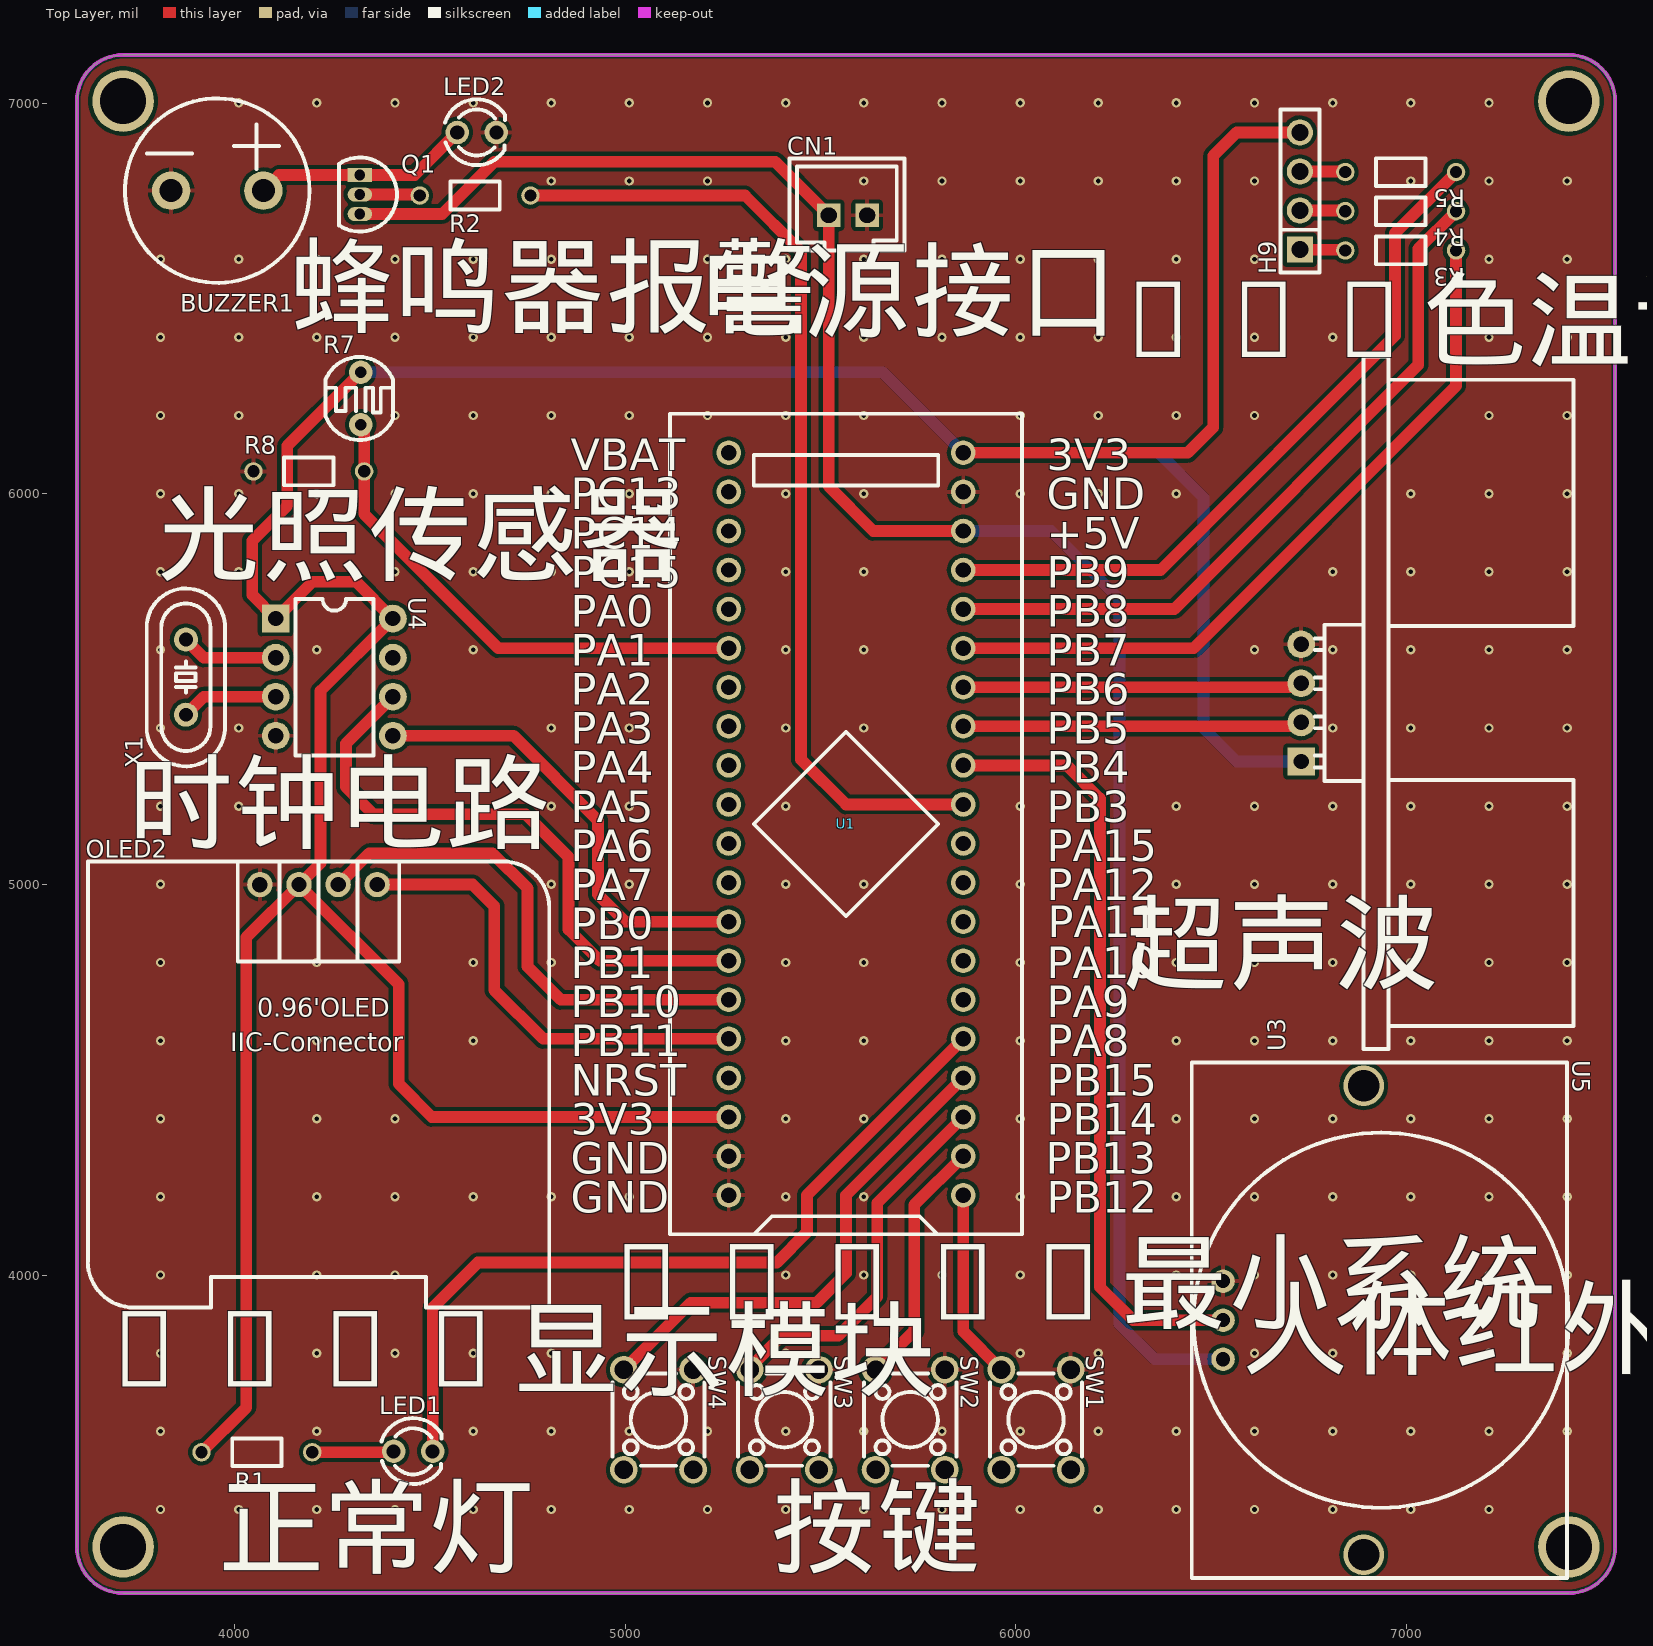
[diagram p0: Top Layer view]
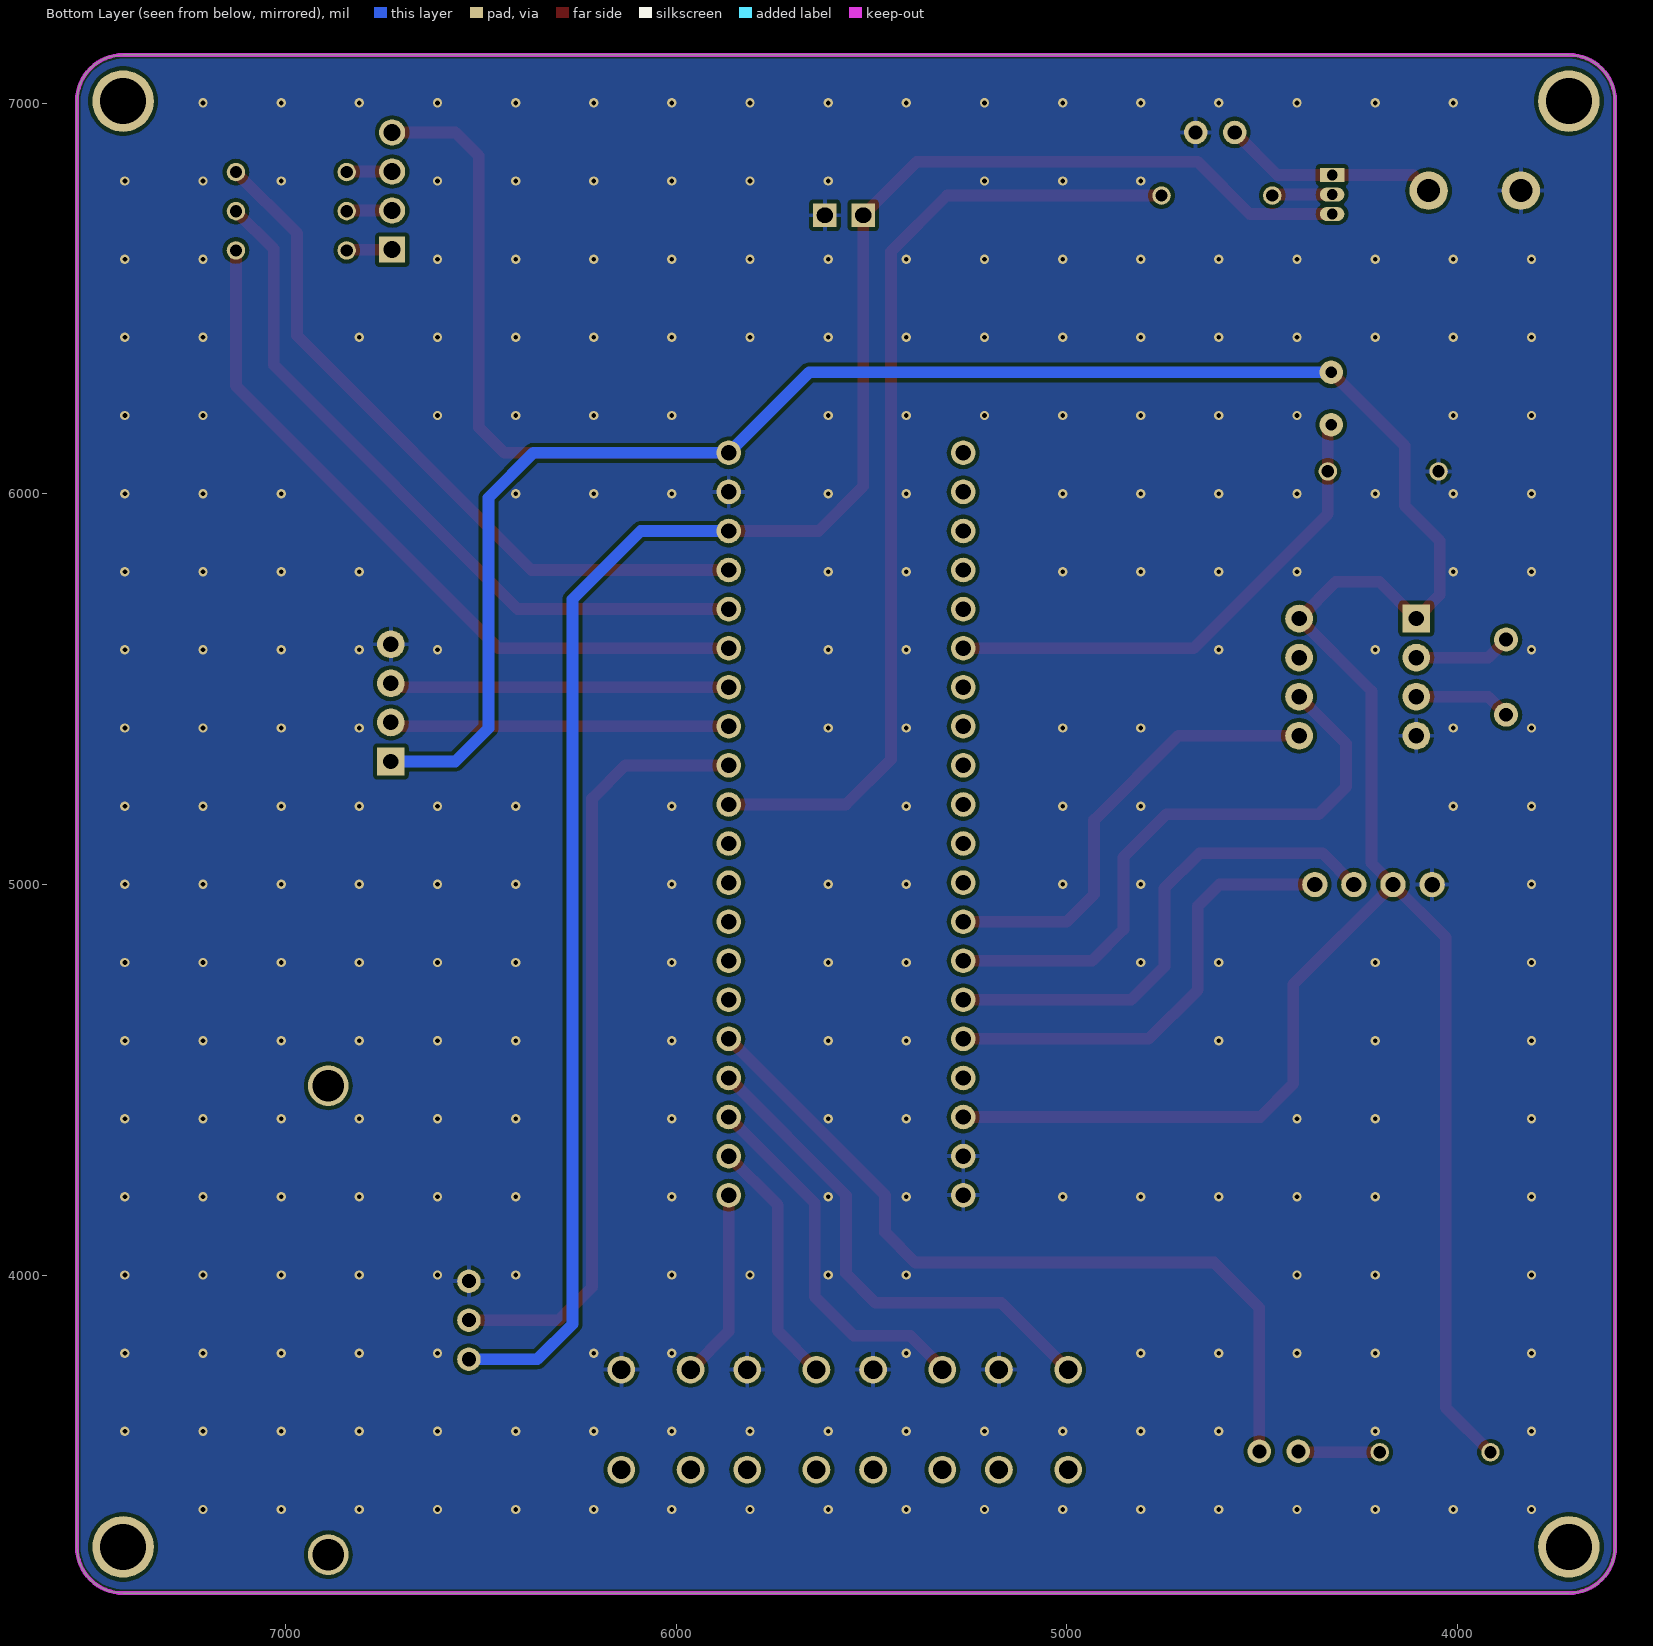
[diagram p1: Bottom Layer view, seen from below]
# Altium PCB MISC51867.pcbdoc
Units mil, origin at the board's own origin, x right, y up, seen from the top; angles counter-clockwise.
Board outline 3937.01 x 3937.01 mil, 2 copper layers (Top Layer, Bottom Layer), stack 62.206 mil thick; 23 components, 46 nets, 112 pads, 263 vias.

## Layer stack, top to bottom
Top Solder Mask Layer: solder mask 0.394, Dk 3.3
Top Layer: signal copper 1.379
Dielectric1: surface 59.449, FR4, Dk 4.5
Bottom Layer: signal copper 1.378
Bottom Solder Mask Layer: solder mask 0.394, Dk 3.3

## Board outline
3714.61,7123.5 ccw(c3714.61,7005.39) 3596.5,7005.39 3596.5,3304.61 ccw(c3714.61,3304.61) 3714.61,3186.5 7415.39,3186.5 ccw(c7415.39,3304.61) 7533.5,3304.61 7533.5,7005.39 ccw(c7415.39,7005.39) 7415.39,7123.5 3714.61,7123.5

## Design rules (kind name [scope] priority, off if disabled: settings)
BoardOutlineClearance copperThickness2oz_1 [All] p2 off: genericclearance=7.99 ignorepadtopadclearanceinfootprint=FALSE except(0: Arc-SplitContinuation Track-SplitContinuation SMDPad-SplitContinuation THPad-SplitContinuation Via-SplitContinuation Fill-SplitContinuation Region-SplitContinuation Poly-SplitContinuation Text-SplitContinuation Hole-SplitContinuation; 5.98: Arc-CutoutEdge Track-CutoutEdge SMDPad-CutoutEdge THPad-CutoutEdge Via-CutoutEdge Text-CutoutEdge; 6.9: Hole-OutlineEdge Hole-CutoutEdge; 10: Poly-OutlineEdge Poly-CutoutEdge; 11.81: Arc-OutlineEdge Track-OutlineEdge SMDPad-OutlineEdge THPad-OutlineEdge Via-OutlineEdge Fill-OutlineEdge Region-OutlineEdge Text-OutlineEdge Fill-CutoutEdge Region-CutoutEdge)
BoardOutlineClearance Plane_innerPlane_1 [All] p4 off: genericclearance=4.02 ignorepadtopadclearanceinfootprint=FALSE except(0: Arc-SplitContinuation Track-SplitContinuation SMDPad-SplitContinuation THPad-SplitContinuation Via-SplitContinuation Fill-SplitContinuation Region-SplitContinuation Poly-SplitContinuation Text-SplitContinuation Hole-SplitContinuation; 5.98: Arc-CutoutEdge Track-CutoutEdge SMDPad-CutoutEdge THPad-CutoutEdge Via-CutoutEdge Text-CutoutEdge; 6.9: Hole-OutlineEdge Hole-CutoutEdge; 10: Poly-OutlineEdge Poly-CutoutEdge; 11.81: Arc-OutlineEdge Track-OutlineEdge SMDPad-OutlineEdge THPad-OutlineEdge Via-OutlineEdge Fill-OutlineEdge Region-OutlineEdge Text-OutlineEdge Fill-CutoutEdge Region-CutoutEdge)
BoardOutlineClearance Copper_copperRegion_1 [All] p6 off: genericclearance=4.02 ignorepadtopadclearanceinfootprint=FALSE except(0: Arc-SplitContinuation Track-SplitContinuation SMDPad-SplitContinuation THPad-SplitContinuation Via-SplitContinuation Fill-SplitContinuation Region-SplitContinuation Poly-SplitContinuation Text-SplitContinuation Hole-SplitContinuation; 5.98: Arc-CutoutEdge Track-CutoutEdge SMDPad-CutoutEdge THPad-CutoutEdge Via-CutoutEdge Text-CutoutEdge; 6.9: Hole-OutlineEdge Hole-CutoutEdge; 10: Poly-OutlineEdge Poly-CutoutEdge; 11.81: Arc-OutlineEdge Track-OutlineEdge SMDPad-OutlineEdge THPad-OutlineEdge Via-OutlineEdge Fill-OutlineEdge Region-OutlineEdge Text-OutlineEdge Fill-CutoutEdge Region-CutoutEdge)
BoardOutlineClearance Copper_copperRegion_copperThickness1oz_1 [All] p8 off: genericclearance=4.02 ignorepadtopadclearanceinfootprint=FALSE except(0: Arc-SplitContinuation Track-SplitContinuation SMDPad-SplitContinuation THPad-SplitContinuation Via-SplitContinuation Fill-SplitContinuation Region-SplitContinuation Poly-SplitContinuation Text-SplitContinuation Hole-SplitContinuation; 5.98: Arc-CutoutEdge Track-CutoutEdge SMDPad-CutoutEdge THPad-CutoutEdge Via-CutoutEdge Text-CutoutEdge; 6.9: Hole-OutlineEdge Hole-CutoutEdge; 10: Poly-OutlineEdge Poly-CutoutEdge; 11.81: Arc-OutlineEdge Track-OutlineEdge SMDPad-OutlineEdge THPad-OutlineEdge Via-OutlineEdge Fill-OutlineEdge Region-OutlineEdge Text-OutlineEdge Fill-CutoutEdge Region-CutoutEdge)
BoardOutlineClearance Copper_copperRegion_Copper_copperRegion_1 [All] p10 off: genericclearance=4.02 ignorepadtopadclearanceinfootprint=FALSE except(0: Arc-SplitContinuation Track-SplitContinuation SMDPad-SplitContinuation THPad-SplitContinuation Via-SplitContinuation Fill-SplitContinuation Region-SplitContinuation Poly-SplitContinuation Text-SplitContinuation Hole-SplitContinuation; 5.98: Arc-CutoutEdge Track-CutoutEdge SMDPad-CutoutEdge THPad-CutoutEdge Via-CutoutEdge Text-CutoutEdge; 6.9: Hole-OutlineEdge Hole-CutoutEdge; 10: Poly-OutlineEdge Poly-CutoutEdge; 11.81: Arc-OutlineEdge Track-OutlineEdge SMDPad-OutlineEdge THPad-OutlineEdge Via-OutlineEdge Fill-OutlineEdge Region-OutlineEdge Text-OutlineEdge Fill-CutoutEdge Region-CutoutEdge)
BoardOutlineClearance copperThickness1oz_1 [All] p12: genericclearance=4.02 ignorepadtopadclearanceinfootprint=FALSE except(0: Arc-SplitContinuation Track-SplitContinuation SMDPad-SplitContinuation THPad-SplitContinuation Via-SplitContinuation Fill-SplitContinuation Region-SplitContinuation Poly-SplitContinuation Text-SplitContinuation Hole-SplitContinuation; 5.98: Arc-CutoutEdge Track-CutoutEdge SMDPad-CutoutEdge THPad-CutoutEdge Via-CutoutEdge Text-CutoutEdge; 6.9: Hole-OutlineEdge Hole-CutoutEdge; 10: Poly-OutlineEdge Poly-CutoutEdge; 11.81: Arc-OutlineEdge Track-OutlineEdge SMDPad-OutlineEdge THPad-OutlineEdge Via-OutlineEdge Fill-OutlineEdge Region-OutlineEdge Text-OutlineEdge Fill-CutoutEdge Region-CutoutEdge)
Clearance copperThickness2oz [All] p1 off: gap=7.99 ignorepadtopadclearanceinfootprint=FALSE except(5.98: SMDPad-Track SMDPad-SMDPad THPad-Track SMDPad-THPad THPad-THPad Track-Via SMDPad-Via THPad-Via Via-Via Fill-SMDPad Region-SMDPad Fill-THPad Region-THPad Fill-Via Region-Via Fill-Fill Fill-Region Region-Region Arc-Track Arc-SMDPad Arc-THPad Arc-Via Fill-Arc Region-Arc Arc-Arc Text-Track SMDPad-Text Text-THPad Text-Via Fill-Text Region-Text Arc-Text Text-Text; 6.9: Hole-Track Hole-SMDPad Hole-THPad Hole-Via Fill-Hole Region-Hole Hole-Arc Hole-Text; 10: Poly-Track Poly-SMDPad Poly-THPad Poly-Via Poly-Fill Poly-Region Poly-Poly Poly-Arc Poly-Text Poly-Hole; 11.81: Fill-Track Region-Track)
Clearance Plane_innerPlane [All] p3 off: gap=4.02 ignorepadtopadclearanceinfootprint=FALSE except(5.98: SMDPad-Track SMDPad-SMDPad THPad-Track SMDPad-THPad THPad-THPad Track-Via SMDPad-Via THPad-Via Via-Via Fill-SMDPad Region-SMDPad Fill-THPad Region-THPad Fill-Via Region-Via Fill-Fill Fill-Region Region-Region Arc-Track Arc-SMDPad Arc-THPad Arc-Via Fill-Arc Region-Arc Arc-Arc Text-Track SMDPad-Text Text-THPad Text-Via Fill-Text Region-Text Arc-Text Text-Text; 6.9: Hole-Track Hole-SMDPad Hole-THPad Hole-Via Fill-Hole Region-Hole Hole-Arc Hole-Text; 10: Poly-Track Poly-SMDPad Poly-THPad Poly-Via Poly-Fill Poly-Region Poly-Poly Poly-Arc Poly-Text Poly-Hole; 11.81: Fill-Track Region-Track)
Clearance Copper_copperRegion [All] p5 off: gap=4.02 ignorepadtopadclearanceinfootprint=FALSE except(5.98: SMDPad-Track SMDPad-SMDPad THPad-Track SMDPad-THPad THPad-THPad Track-Via SMDPad-Via THPad-Via Via-Via Fill-SMDPad Region-SMDPad Fill-THPad Region-THPad Fill-Via Region-Via Fill-Fill Fill-Region Region-Region Arc-Track Arc-SMDPad Arc-THPad Arc-Via Fill-Arc Region-Arc Arc-Arc Text-Track SMDPad-Text Text-THPad Text-Via Fill-Text Region-Text Arc-Text Text-Text; 6.9: Hole-Track Hole-SMDPad Hole-THPad Hole-Via Fill-Hole Region-Hole Hole-Arc Hole-Text; 10: Poly-Track Poly-SMDPad Poly-THPad Poly-Via Poly-Fill Poly-Region Poly-Poly Poly-Arc Poly-Text Poly-Hole; 11.81: Fill-Track Region-Track)
Clearance Copper_copperRegion_copperThickness1oz [All] p7 off: gap=4.02 ignorepadtopadclearanceinfootprint=FALSE except(5.98: SMDPad-Track SMDPad-SMDPad THPad-Track SMDPad-THPad THPad-THPad Track-Via SMDPad-Via THPad-Via Via-Via Fill-SMDPad Region-SMDPad Fill-THPad Region-THPad Fill-Via Region-Via Fill-Fill Fill-Region Region-Region Arc-Track Arc-SMDPad Arc-THPad Arc-Via Fill-Arc Region-Arc Arc-Arc Text-Track SMDPad-Text Text-THPad Text-Via Fill-Text Region-Text Arc-Text Text-Text; 6.9: Hole-Track Hole-SMDPad Hole-THPad Hole-Via Fill-Hole Region-Hole Hole-Arc Hole-Text; 10: Poly-Track Poly-SMDPad Poly-THPad Poly-Via Poly-Fill Poly-Region Poly-Poly Poly-Arc Poly-Text Poly-Hole; 11.81: Fill-Track Region-Track)
Clearance Copper_copperRegion_Copper_copperRegion [All] p9 off: gap=4.02 ignorepadtopadclearanceinfootprint=FALSE except(5.98: SMDPad-Track SMDPad-SMDPad THPad-Track SMDPad-THPad THPad-THPad Track-Via SMDPad-Via THPad-Via Via-Via Fill-SMDPad Region-SMDPad Fill-THPad Region-THPad Fill-Via Region-Via Fill-Fill Fill-Region Region-Region Arc-Track Arc-SMDPad Arc-THPad Arc-Via Fill-Arc Region-Arc Arc-Arc Text-Track SMDPad-Text Text-THPad Text-Via Fill-Text Region-Text Arc-Text Text-Text; 6.9: Hole-Track Hole-SMDPad Hole-THPad Hole-Via Fill-Hole Region-Hole Hole-Arc Hole-Text; 10: Poly-Track Poly-SMDPad Poly-THPad Poly-Via Poly-Fill Poly-Region Poly-Poly Poly-Arc Poly-Text Poly-Hole; 11.81: Fill-Track Region-Track)
Clearance copperThickness1oz [All] p11: gap=4.02 ignorepadtopadclearanceinfootprint=FALSE except(5.98: SMDPad-Track SMDPad-SMDPad THPad-Track SMDPad-THPad THPad-THPad Track-Via SMDPad-Via THPad-Via Via-Via Fill-SMDPad Region-SMDPad Fill-THPad Region-THPad Fill-Via Region-Via Fill-Fill Fill-Region Region-Region Arc-Track Arc-SMDPad Arc-THPad Arc-Via Fill-Arc Region-Arc Arc-Arc Text-Track SMDPad-Text Text-THPad Text-Via Fill-Text Region-Text Arc-Text Text-Text; 6.9: Hole-Track Hole-SMDPad Hole-THPad Hole-Via Fill-Hole Region-Hole Hole-Arc Hole-Text; 10: Poly-Track Poly-SMDPad Poly-THPad Poly-Via Poly-Fill Poly-Region Poly-Poly Poly-Arc Poly-Text Poly-Hole; 11.81: Fill-Track Region-Track)
DiffPairsRouting differentialPair [All] p1: maxlimit=6 minlimit=6 mostfreqgap=6 toplayer_minwidth=5 toplayer_prefwidth=10 toplayer_maxwidth=100 toplayer_mingap=6 toplayer_prefgap=6 toplayer_maxgap=6 bottomlayer_minwidth=5 bottomlayer_prefwidth=10 bottomlayer_maxwidth=100 bottomlayer_mingap=6 bottomlayer_prefgap=6 bottomlayer_maxgap=6 maxuncoupledlength=10
HoleToHoleClearance otherClearance [All] p1: gap=11.81 allowstackedmicrovias=TRUE
Length netLength [All] p1: minlimit=0 maxlimit=0
PasteMaskExpansion pasteMaskExpansion [All] p1: expansion=0
PlaneConnect innerPlane [All] p1: planeconnectstyle=Relief reliefexpansion=20 reliefentries=4 reliefconductorwidth=10 reliefairgap=10
PolygonConnect copperRegion_copperThickness1oz [All] p1 off: connectstyle=Relief reliefconductorwidth=10 reliefentries=4 polygonreliefangle="90 Angle" airgapwidth=10 via.connectstyle=Relief via.reliefconductorwidth=10 via.reliefentries=4 via.polygonreliefangle="90 Angle" via.airgapwidth=10
PolygonConnect copperRegion_Copper_copperRegion [All] p2 off: connectstyle=Relief reliefconductorwidth=10 reliefentries=4 polygonreliefangle="90 Angle" airgapwidth=10 via.connectstyle=Relief via.reliefconductorwidth=10 via.reliefentries=4 via.polygonreliefangle="90 Angle" via.airgapwidth=10
PolygonConnect copperRegion [All] p3: connectstyle=Relief reliefconductorwidth=10 reliefentries=4 polygonreliefangle="90 Angle" airgapwidth=10 via.connectstyle=Relief via.reliefconductorwidth=10 via.reliefentries=4 via.polygonreliefangle="90 Angle" via.airgapwidth=10
RoutingVias viaSize [All] p1: holewidth=12.01 width=24.02 viastyle="Through Hole" minholewidth=11.81 minwidth=19.68 maxholewidth=248.03 maxwidth=393.7
SolderMaskExpansion solderMaskExpansion [IsVia] p1: expansion=-1000 istentingtop=TRUE
SolderMaskExpansion solderMaskExpansion [All] p2: expansion=2 istentingtop=FALSE
Width copperThickness2oz_2 [All] p1 off: maxlimit=100 minlimit=8 preferedwidth=10
Width copperThickness1oz_2 [All] p2: maxlimit=100 minlimit=5 preferedwidth=10

## Components (designator, comment, footprint, x,y, rotation, side; value= is the part's Value field where it differs from the comment)
BUZZER1 "buzzer" BUZ-TH_BD12.0-P6.00-D0.9-RD 3955.71,6776.01 r0 top
CN1 "XH2.54-2PIN-直针" CONN-TH_XH2.54-2P 5569.9,6713.05 r0 top
H9 "" HDR-TH_4P-P2.54-V-F 6726.57,6775 r90 top
LED1 "" LED_TH-3mm 4457.17,3549.42 r0 top
LED2 "" LED_TH-3mm 4620,6925 r0 top
OLED2 "" 0.96OLED_4P 4215,5000 r0 top
Q1 "" S8050_TO_92 4320.71,6766.01 r270 top
R1 "10kΩ" Res_1/8W 4057.17,3549.42 r180 top
R2 "1kΩ" Res_1/8W 4615.71,6766.01 r180 top
R3 "100Ω" Res_1/8W 6984.7,6625.52 r180 top
R4 "100Ω" Res_1/8W 6984.7,6726.01 r180 top
R5 "100Ω" Res_1/8W 6984.7,6826.01 r180 top
R7 "GL5549(80-100)" RES-TH_L5.1-W4.3-P3.40-D0.5 4323.15,6243.99 r0 top
R8 "10kΩ" Res_1/8W 4190,6055 r0 top
SW1 "" SW-TH_4P-L6.0-W6.0-P4.50-LS6.5 6051.36,3630.47 r270 top
SW2 "" SW-TH_4P-L6.0-W6.0-P4.50-LS6.5 5729.24,3630.47 r270 top
SW3 "" SW-TH_4P-L6.0-W6.0-P4.50-LS6.5 5407.12,3630.47 r270 top
SW4 "" SW-TH_4P-L6.0-W6.0-P4.50-LS6.5 5085,3630.47 r270 top
U1 "STM32F103C8T6-Card" CONN-TH_L53.3-W22.9_STM32F103C8T6-CARD 5565,5155 r90 top
U3 "HC-SR04" TH_HC-SR04V 6730,5465 r90 top
U4 "DS1302N" DIP-8_L9.7-W6.4-P2.54-LS7.6-BL 4255.41,5530.83 r270 top
U5 "" HC-SR501 6930,3885 r270 top
X1 "32.768KHZ" HC-49S_L11.5-W5.0-P4.88 3875.41,5530.83 r90 top

## Footprints (in the part's own frame and the unit in brackets; to place one, negate y for a bottom-side part, rotate by r counter-clockwise, add the part's x,y. Pads: shape width x height; smd on the part's side, far side on the other; paste and mask are expansions set on the pad)
0.96OLED_4P [mm]
  round 1.65 hole 1 copper offset 0,0: 1(-3.81,-0.001) 2(-1.27,0.002) 3(1.27,0.002) 4(3.81,0.002)
  silkscreen extent -15,-27.5 15,1.5
BUZ-TH_BD12.0-P6.00-D0.9-RD [mm]
  round 2.5 hole 1.5 paste+0 mask+0.05: 1(-3,0) 2(3,0)
  silkscreen extent -5.99,-5.99 5.99,5.99
CONN-TH_L53.3-W22.9_STM32F103C8T6-CARD [mm]
  round 1.6 hole 1: 1(-24.13,-7.62) 2(-21.59,-7.62) 3(-19.05,-7.62) 4(-16.51,-7.62) 5(-13.97,-7.62) 6(-11.43,-7.62) 7(-8.89,-7.62) 8(-6.35,-7.62) 9(-3.81,-7.62) 10(-1.27,-7.62) 11(1.27,-7.62) 12(3.81,-7.62) 13(6.35,-7.62) 14(8.89,-7.62) 15(11.43,-7.62) 16(13.97,-7.62) 17(16.51,-7.62) 18(19.05,-7.62) 19(21.59,-7.62) 20(24.13,-7.62) 21(24.13,7.62) 22(21.59,7.62) 23(19.05,7.62) 24(16.51,7.62) 25(13.97,7.62) 26(11.43,7.62) 27(8.89,7.62) 28(6.35,7.62) 29(3.81,7.62) 30(1.27,7.62) 31(-1.27,7.62) 32(-3.81,7.62) 33(-6.35,7.62) 34(-8.89,7.62) 35(-11.43,7.62) 36(-13.97,7.62) 37(-16.51,7.62) 38(-19.05,7.62) 39(-21.59,7.62) 40(-24.13,7.62)
  silkscreen extent -26.67,-11.43 26.67,11.43
CONN-TH_XH2.54-2P [mil]
  rect 60x60 hole 39.37 slot 41.34 at 0 deg paste+0 mask+1.97: 1(-49.22,0) 2(49.21,0)
  silkscreen extent -150,-90 145,145
DIP-8_L9.7-W6.4-P2.54-LS7.6-BL [mm]
  rect 1.8x1.8 hole 1 paste+0 mask+0.05: 1(-3.81,-3.81)
  round 1.8 hole 1 paste+0 mask+0.05: 2(-1.27,-3.81) 3(1.27,-3.81) 4(3.81,-3.81) 5(3.81,3.81) 6(1.27,3.81) 7(-1.27,3.81) 8(-3.81,3.81)
  silkscreen extent -5.08,-2.53 5.08,2.53
HC-49S_L11.5-W5.0-P4.88 [mm]
  round 1.56 hole 0.9: 1(-2.44,0) 2(2.44,0)
  silkscreen extent -5.8,-2.54 5.77,2.54
HC-SR501 [mil]
  round 60 hole 35.98: 1(-100,-400) 2(0,-400) 3(100,-400)
  round 104.02 hole 80: ""(-600,-40) ""(600,-40)
  silkscreen extent -660,-480 660,485
HDR-TH_4P-P2.54-V-F [mm]
  rect 1.7x1.7 hole 1.1: 1(-3.81,0)
  round 1.7 hole 1.1: 2(-1.27,0) 3(1.27,0) 4(3.81,0)
  silkscreen extent -5.29,-1.27 5.29,1.27
LED_TH-3mm [mil]
  round 60 hole 36 paste+0 mask+2: 1(-50,0) 2(50,0)
  silkscreen extent -81,-84 72,85
RES-TH_L5.1-W4.3-P3.40-D0.5 [mil]
  round 60 hole 30: 1(0,66.93) 2(0,-66.93)
  silkscreen extent -91,-106 83,106
Res_1/8W [mil]
  round 47.2 hole 31.5 paste+0 mask+2: 1(-141.7,2.48) 2(141.7,2.48)
  silkscreen extent -63,-33 63,38
S8050_TO_92 [mil]
  rect 35.4x63 hole 27.6 paste+0 mask+2: 1(-50,0)
  oval 35.4x63 hole 27.6 paste+0 mask+2: 2(0,0) 3(50,0)
  silkscreen extent -95,-53 95,95
SW-TH_4P-L6.0-W6.0-P4.50-LS6.5 [mm]
  round 1.8 hole 1.2: 1(-3.25,2.25) 2(3.25,2.25) 3(-3.25,-2.25) 4(3.25,-2.25)
  silkscreen extent -3,-3 3,3
TH_HC-SR04V [mm]
  rect 1.8x1.8 hole 1.001: 1(-3.81,0)
  round 1.8 hole 1.001: 2(-1.27,0) 3(1.27,0) 4(3.81,0)
  silkscreen extent -22.5,-17.7 22.5,-0.89

## Free pads (board coordinates)
  round 157.48 hole 118.11: 1(3714.61,7005.39) 1(3714.61,3304.61) 1(7415.39,7005.39) 1(7415.39,3304.61)

## Via types
v1: diameter 24.02, hole 12, Top Layer to Bottom Layer, 263 vias

## Nets (pads, with @x,y where several pads share a name; then routed paths per layer and width w, separated by ;. In a path a pad name is that pad's centre, name@x,y a point inside that pad or via, vN(x,y) a via of type N, cw(c..) or ccw(c..) an arc to the next point about the centre after c; other vN are vias at no path point)
$1N17250: Q1.2 R2.2 | length 154.3
  Top Layer w30: Q1.2 4471.53,6766.01 R2.2
$1N17251: BUZZER1.2 LED2.1 Q1.1 | length 557.9
  Top Layer w30: BUZZER1.2 4113.82,6816.01 Q1.1 4461.01,6816.01 LED2.1
$1N17254: H9.1 R3.2 | length 117.2
  Top Layer w30: H9.1 6841.05,6625 R3.2
$1N17257: H9.2 R4.2 | length 117
  Top Layer w30: H9.2 6841.53,6725 R4.2
$1N17259: H9.3 R5.2 | length 117
  Top Layer w30: H9.3 6841.53,6825 R5.2
$1N17263: LED1.1 R1.1 | length 209.3
  Top Layer w30: R1.1 4404.7,3546.94 LED1.1
$1N17264: U4.2 X1.2 | length 249.1
  Top Layer w30: X1.2 3921.47,5580.83 U4.2
$1N17265: U4.3 X1.1 | length 249.1
  Top Layer w30: X1.1 3921.47,5480.83 U4.3
+5V: CN1.1 Q1.3 U1.18 U5.3 | length 5027.4
  Top Layer w30: Q1.3 4531.01,6716.01 4665,6850 5383.74,6850 CN1.1 5520.69,6019.31 5635,5905 U1.18
  Bottom Layer w30: U1.18 6090,5905 6265,5730 6265,3875 6355,3785 U5.3
GND: BUZZER1.1 CN1.2 LED2.2 OLED2.1 R8.1 SW1.1 SW2.1 SW3.1 SW4.1 U1.19 U1.39 U1.40 U3.4 U4.4 U5.1
  other v1: 3810.6,3400.6 4010.6,3400.6 4210.6,3400.6 4410.6,3400.6 4610.6,3400.6 4810.6,3400.6 5010.6,3400.6 5210.6,3400.6 5410.6,3400.6 5610.6,3400.6 5810.6,3400.6 6010.6,3400.6 6210.6,3400.6 6410.6,3400.6 6610.6,3400.6 6810.6,3400.6 7010.6,3400.6 7210.6,3400.6 3810.6,3600.6 4210.6,3600.6 4610.6,3600.6 4810.6,3600.6 5010.6,3600.6 5210.6,3600.6 5410.6,3600.6 5610.6,3600.6 5810.6,3600.6 6010.6,3600.6 6210.6,3600.6 6410.6,3600.6 6610.6,3600.6 6810.6,3600.6 7010.6,3600.6 7210.6,3600.6 7410.6,3600.6 3810.6,3800.6 4210.6,3800.6 4410.6,3800.6 4610.6,3800.6 4810.6,3800.6 5410.6,3800.6 6010.6,3800.6 6210.6,3800.6 6610.6,3800.6 6810.6,3800.6 7010.6,3800.6 7210.6,3800.6 7410.6,3800.6 3810.6,4000.6 4210.6,4000.6 4410.6,4000.6 5410.6,4000.6 5610.6,4000.6 5810.6,4000.6 6010.6,4000.6 6410.6,4000.6 6610.6,4000.6 6810.6,4000.6 7010.6,4000.6 7210.6,4000.6 7410.6,4000.6 3810.6,4200.6 4210.6,4200.6 4410.6,4200.6 4610.6,4200.6 4810.6,4200.6 5010.6,4200.6 5410.6,4200.6 5610.6,4200.6 6010.6,4200.6 6410.6,4200.6 6610.6,4200.6 6810.6,4200.6 7010.6,4200.6 7210.6,4200.6 7410.6,4200.6 3810.6,4400.6 4210.6,4400.6 4410.6,4400.6 5410.6,4400.6 5610.6,4400.6 6010.6,4400.6 6410.6,4400.6 6610.6,4400.6 6810.6,4400.6 7010.6,4400.6 7210.6,4400.6 7410.6,4400.6 3810.6,4600.6 4210.6,4600.6 4610.6,4600.6 5410.6,4600.6 5610.6,4600.6 6010.6,4600.6 6410.6,4600.6 6610.6,4600.6 6810.6,4600.6 7010.6,4600.6 7210.6,4600.6 7410.6,4600.6 3810.6,4800.6 4210.6,4800.6 4610.6,4800.6 4810.6,4800.6 5410.6,4800.6 5610.6,4800.6 6010.6,4800.6 6410.6,4800.6 6610.6,4800.6 6810.6,4800.6 7010.6,4800.6 7210.6,4800.6 7410.6,4800.6 3810.6,5000.6 4810.6,5000.6 5010.6,5000.6 5410.6,5000.6 5610.6,5000.6 6010.6,5000.6 6410.6,5000.6 6610.6,5000.6 6810.6,5000.6 7010.6,5000.6 7210.6,5000.6 7410.6,5000.6 3810.6,5200.6 4010.6,5200.6 4810.6,5200.6 5010.6,5200.6 5410.6,5200.6 6010.6,5200.6 6410.6,5200.6 6610.6,5200.6 6810.6,5200.6 7010.6,5200.6 7210.6,5200.6 7410.6,5200.6 3810.6,5400.6 4010.6,5400.6 4810.6,5400.6 5010.6,5400.6 5410.6,5400.6 5610.6,5400.6 6810.6,5400.6 7010.6,5400.6 7210.6,5400.6 7410.6,5400.6 3810.6,5600.6 4210.6,5600.6 4610.6,5600.6 5410.6,5600.6 5610.6,5600.6 6610.6,5600.6 6810.6,5600.6 7010.6,5600.6 7210.6,5600.6 7410.6,5600.6 3810.6,5800.6 4010.6,5800.6 4410.6,5800.6 4610.6,5800.6 4810.6,5800.6 5010.6,5800.6 5410.6,5800.6 5610.6,5800.6 6810.6,5800.6 7010.6,5800.6 7210.6,5800.6 7410.6,5800.6 3810.6,6000.6 4010.6,6000.6 4210.6,6000.6 4410.6,6000.6 4610.6,6000.6 4810.6,6000.6 5010.6,6000.6 5410.6,6000.6 5610.6,6000.6 6010.6,6000.6 6210.6,6000.6 6410.6,6000.6 7010.6,6000.6 7210.6,6000.6 7410.6,6000.6 3810.6,6200.6 4010.6,6200.6 4410.6,6200.6 4610.6,6200.6 4810.6,6200.6 5010.6,6200.6 5210.6,6200.6 5410.6,6200.6 5610.6,6200.6 6010.6,6200.6 6210.6,6200.6 6410.6,6200.6 6610.6,6200.6 7210.6,6200.6 7410.6,6200.6 3810.6,6400.6 4010.6,6400.6 4210.6,6400.6 4410.6,6400.6 4610.6,6400.6 4810.6,6400.6 5010.6,6400.6 5210.6,6400.6 5410.6,6400.6 5610.6,6400.6 5810.6,6400.6 6010.6,6400.6 6210.6,6400.6 6410.6,6400.6 6610.6,6400.6 6810.6,6400.6 7210.6,6400.6 7410.6,6400.6 3810.6,6600.6 4010.6,6600.6 4210.6,6600.6 4410.6,6600.6 4610.6,6600.6 4810.6,6600.6 5010.6,6600.6 5210.6,6600.6 5410.6,6600.6 5610.6,6600.6 5810.6,6600.6 6010.6,6600.6 6210.6,6600.6 6410.6,6600.6 6610.6,6600.6 7210.6,6600.6 7410.6,6600.6 4810.6,6800.6 5010.6,6800.6 5210.6,6800.6 5610.6,6800.6 5810.6,6800.6 6010.6,6800.6 6210.6,6800.6 6410.6,6800.6 6610.6,6800.6 7010.6,6800.6 7210.6,6800.6 7410.6,6800.6 4010.6,7000.6 4210.6,7000.6 4410.6,7000.6 4610.6,7000.6 4810.6,7000.6 5010.6,7000.6 5210.6,7000.6 5410.6,7000.6 5610.6,7000.6 5810.6,7000.6 6010.6,7000.6 6210.6,7000.6 6410.6,7000.6 6610.6,7000.6 6810.6,7000.6 7010.6,7000.6 7210.6,7000.6
NRST: U1.37
PA0: U1.25
PA1: R7.2 R8.2 U1.26 | length 1307.8
  Top Layer w30: R7.2 4331.7,6168.51 R8.2 4331.7,5948.3 4675,5605 U1.26
PA2: U1.27
PA3: U1.28
PA4: U1.29
PA5: U1.30
PA6: U1.31
PA7: U1.32
PA8: LED1.2 U1.5 | length 2066.1
  Top Layer w30: LED1.2 4507.17,3917.17 4622.5,4032.5 5387.5,4032.5 5465,4110 5465,4205 U1.5
PA9: U1.6
PA10: U1.7
PA11: U1.8
PA12: U1.9
PA15: U1.10
PB0: U1.33 U4.5 | length 1168
  Top Layer w30: U4.5 4714.17,5380.83 4930,5165 4930,4975 5000,4905 U1.33
PB1: U1.34 U4.6 | length 1553.4
  Top Layer w30: U4.6 4285,5360.42 4285,5250 4355,5180 4745,5180 4855,5070 4855,4885 4935,4805 U1.34
PB2: U4.7
PB3: R2.1 U1.11 | length 2514.7
  Top Layer w30: R2.1 5306.47,6763.53 5450,6620 5450,5320 5565,5205 U1.11
PB4: U1.12 U5.2 | length 1985.4
  Top Layer w30: U1.12 6130,5305 6215,5220 6215,3970 6300,3885 U5.2
PB5: U1.13 U3.2 | length 869.1
  Top Layer w30: U1.13 6720,5405 U3.2
PB6: U1.14 U3.3 | length 869.1
  Top Layer w30: U1.14 6720,5505 U3.3
PB7: R3.1 U1.15 | length 1886.1
  Top Layer w30: U1.15 6455,5605 7126.4,6276.4 R3.1
PB8: R4.1 U1.16 | length 1857.3
  Top Layer w30: U1.16 6405,5705 7030,6330 7030,6627.13 R4.1
PB9: R5.1 U1.17 | length 1836.8
  Top Layer w30: U1.17 6370,5805 6970,6405 6970,6667.13 R5.1
PB10: OLED2.3 U1.35 | length 1305.6
  Top Layer w30: OLED2.3@4265,5000.05 4344.95,5080 4660,5080 4750,4990 4750,4790 4835,4705 U1.35
PB11: OLED2.4 U1.36 | length 1189.6
  Top Layer w30: OLED2.4@4365,5000.05 4609.95,5000.05 4665,4945 4665,4730 4790,4605 U1.36
PB12: SW1.3 U1.1 | length 487.1
  Top Layer w30: U1.1 5865,3856.2 SW1.3
PB13: SW2.3 U1.2 | length 639.5
  Top Layer w30: SW2.3 5740,3857.76 5740,4180 U1.2
PB14: SW3.3 U1.3 | length 957.9
  Top Layer w30: SW3.3 5318.54,3763.54 5400,3845 5545,3845 5645,3945 5645,4185 U1.3
PB15: SW4.3 U1.4 | length 1295
  Top Layer w30: SW4.3 5168,3930 5490,3930 5565,4005 5565,4205 U1.4
PC13: U1.22
PC14: U1.23
PC15: U1.24
VBAT: U1.21
VCC: H9.4 OLED2.2 R1.2 R7.1 U1.20 U1.38 U3.1 U4.1 U4.8 | length 9754.3
  Top Layer w30: R1.2 4030,3661.47 4030,4865.05 OLED2.2@4165,5000.05 ; R7.1 4135,6122.77 4135,5970 4045,5880 4045,5741.24 U4.1 4199.46,5774.87 4311.37,5774.87 U4.8 4220,5495.42 4220,5055.05 OLED2.2@4165,5000.05 ; U1.38 4505,4405 4420,4490 4420,4745.05 OLED2.2@4165,5000.05 ; U1.20 6440,6105 6505,6170 6505,6865 6565,6925 H9.4
  Bottom Layer w30: R7.1 5659.08,6310.92 U1.20 6365,6105 6480,5990 6480,5400 6565,5315 U3.1
pads on no net: SW1.2 SW1.4 SW2.2 SW2.4 SW3.2 SW3.4 SW4.2 SW4.4 U5.

## Polygon pours and split planes (outlines as drawn)
GND on Bottom Layer (solid, remove dead copper, pour order 2): 3525,7245 3525,3080 7700,3080 7700,7245
GND on Top Layer (solid, remove dead copper, pour order 2): 3000,7415 3000,3000 7930,3000 7930,7415

## Keep-outs
Board Outline Layer:
  the board outline again, w10

## Silkscreen, mask and mechanical layers (free items; w line width, h text height)
Top Silkscreen Layer:
  text "蜂鸣器报警" at 4140,6435 h196.85
  text "电源接口" at 5190,6425 h196.85
  text "RGB色温调节器" at 6230,6350 h196.85
  text "VBAT" at 4860.95,6060 h80
  text "3V3" at 6079.16,6060 h80
  text "PC13" at 4860.95,5960 h80
  text "GND" at 6079.16,5960 h80
  text "PC14" at 4860.95,5860 h80
  text "+5V" at 6079.16,5860 h80
  text "光照传感器" at 3800,5800 h196.85
  text "PC15" at 4860.95,5760 h80
  text "PB9" at 6079.16,5760 h80
  text "PA0" at 4860.95,5660 h80
  text "PB8" at 6079.16,5660 h80
  text "PA1" at 4860.95,5560 h80
  text "PB7" at 6079.16,5560 h80
  text "PA2" at 4860.95,5460 h80
  text "PB6" at 6079.16,5460 h80
  text "PA3" at 4860.95,5360 h80
  text "PB5" at 6079.16,5360 h80
  text "PA4" at 4860.95,5260 h80
  text "PB4" at 6079.16,5260 h80
  text "PA5" at 4860.95,5160 h80
  text "PB3" at 6079.16,5160 h80
  text "时钟电路" at 3730,5115 h196.85
  text "PA6" at 4860.95,5060 h80
  text "PA15" at 6079.16,5060 h80
  text "PA7" at 4860.95,4960 h80
  text "PA12" at 6079.16,4960 h80
  text "PA11" at 6080.95,4865 h80
  text "PB0" at 4860.95,4860 h80
  text "PB1" at 4860.95,4760 h80
  text "PA10" at 6079.16,4760 h80
  text "超声波" at 6275,4755 h196.85
  text "PB10" at 4860.95,4660 h80
  text "PA9" at 6079.16,4660 h80
  text "PB11" at 4860.95,4560 h80
  text "PA8" at 6079.16,4560 h80
  text "NRST" at 4860.95,4460 h80
  text "PB15" at 6079.16,4460 h80
  text "3V3" at 4860.95,4360 h80
  text "PB14" at 6079.16,4360 h80
  text "GND" at 4860.95,4260 h80
  text "PB13" at 6075.95,4260 h80
  text "GND" at 4860.95,4160 h80
  text "PB12" at 6079.16,4160 h80
  text "STM32最小系统" at 4919.45,3886.57 h196.85
  text "人体红外" at 6580,3770 h196.85
  text "OLED显示模块" at 3635,3715 h196.85
  text "按键" at 5373.15,3261.57 h196.85
  text "正常灯" at 3960,3260 h196.85